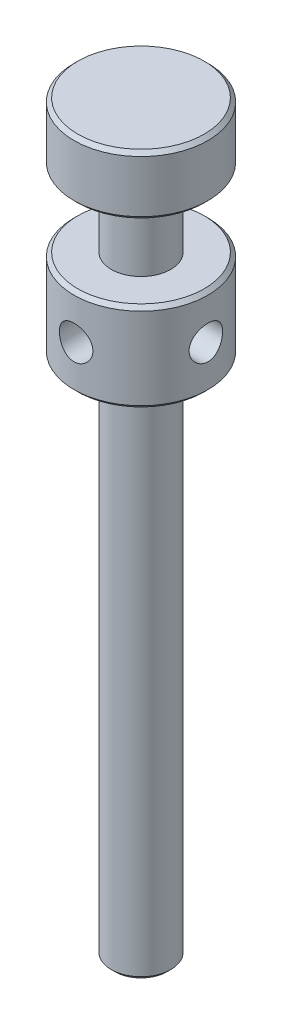
from build123d import *

# Parameters (mm, degrees)
SKETCH1_R           = 4
BOSS_EXTRUDE1_DEPTH = 10
SKETCH2_R           = 9
BOSS_EXTRUDE2_DEPTH = 8
BOSS_EXTRUDE3_START = 12
SKETCH3_R           = 9
BOSS_EXTRUDE3_DEPTH = 12
BOSS_EXTRUDE4_START = 70
SKETCH4_R           = 4
BOSS_EXTRUDE4_DEPTH = 70
CHAMFER1_SIZE       = 0.5
SKETCH6_R           = 2.25
CUT_EXTRUDE2_DEPTH  = 10
CIRPATTERN1_COUNT   = 4
CHAMFER2_SIZE       = 0.5


with BuildPart() as part:
    # Sketch1 → Boss-Extrude1 (new body)
    with BuildSketch(Plane(origin=(0, 0, 0), x_dir=(1, 0, 0), z_dir=(0, 1, 0))):
        with Locations(Location((0, 0, 0), (0, 0, 270))):
            Circle(SKETCH1_R)
    extrude(amount=BOSS_EXTRUDE1_DEPTH)

    # Sketch2 → Boss-Extrude2 (add)
    with BuildSketch(Plane(origin=(0, 10, 0), x_dir=(1, 0, 0), z_dir=(0, 1, 0))):
        with Locations(Location((0, 0, 0), (0, 0, 270))):
            Circle(SKETCH2_R)
    extrude(amount=BOSS_EXTRUDE2_DEPTH)

    # Sketch3 → Boss-Extrude3 (add)
    with BuildSketch(Plane.XZ.offset(BOSS_EXTRUDE3_START)):
        with Locations(Location((0, 0, 0), (0, 0, 90))):
            Circle(SKETCH3_R)
    extrude(amount=-BOSS_EXTRUDE3_DEPTH)

    # Sketch4 → Boss-Extrude4 (add)
    with BuildSketch(Plane.XZ.offset(12).offset(BOSS_EXTRUDE4_START)):
        with Locations(Location((0, 0, 0), (0, 0, 270))):
            Circle(SKETCH4_R)
    extrude(amount=-BOSS_EXTRUDE4_DEPTH)

    # Chamfer1
    chamfer1_edges = [part.edges().sort_by_distance(p)[0] for p in [
        (0, -82, 4),
    ]]
    chamfer(chamfer1_edges, length=CHAMFER1_SIZE)

    # Sketch6 → Cut-Extrude2 (cut)
    with BuildSketch(Plane.XY):
        with Locations((0, -6)):
            Circle(SKETCH6_R)
    cut_extrude2 = extrude(amount=-CUT_EXTRUDE2_DEPTH, mode=Mode.SUBTRACT)

    # CirPattern1: Cut-Extrude2 ×4 about axis
    cirpattern1_axis = Axis((0, 18, 0), (0, -1, 0))
    for i in range(1, CIRPATTERN1_COUNT):
        add(cut_extrude2.rotate(cirpattern1_axis, i * 360 / CIRPATTERN1_COUNT), mode=Mode.SUBTRACT)

    # Chamfer2
    chamfer2_edges = [part.edges().sort_by_distance(p)[0] for p in [
        (0, 10, -9),
        (0, 18, -9),
        (0, 0, -9),
        (0, -12, -9),
    ]]
    chamfer(chamfer2_edges, length=CHAMFER2_SIZE)


solid = part.part
